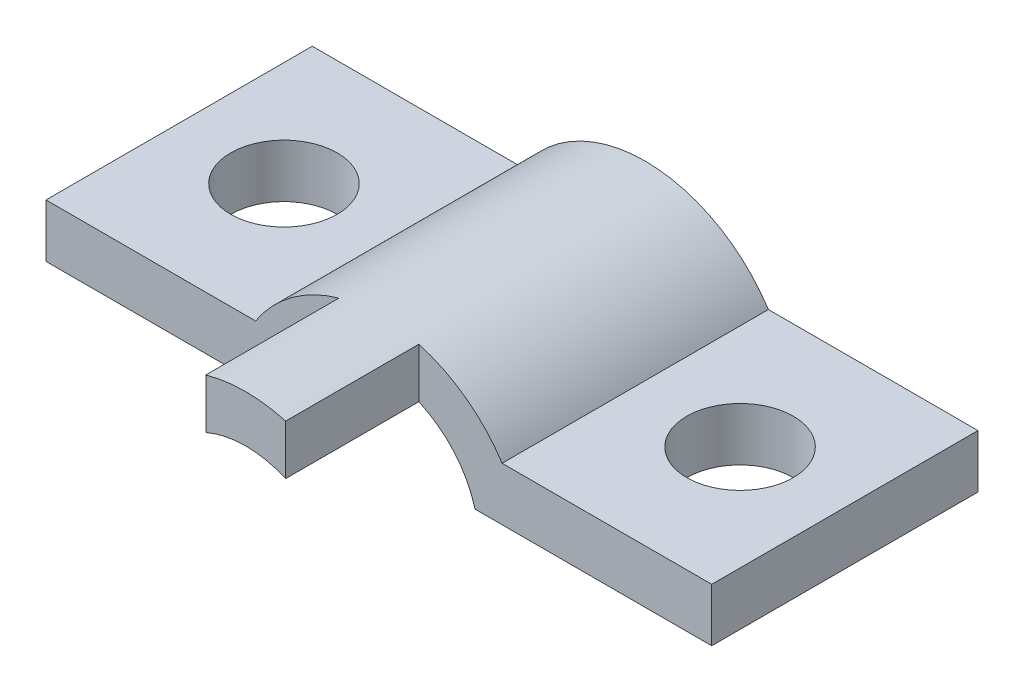
SolidWorks part; units mm, degrees
ref_plane "前视基准面" through (0, 0, 0) normal (0, 0, 1) x (1, 0, 0)
ref_plane "上视基准面" through (0, 0, 0) normal (0, 1, 0) x (1, 0, 0)
ref_plane "右视基准面" through (0, 0, 0) normal (1, 0, 0) x (0, 0, -1)
sketch "草图1" plane through (0, 0, 0) normal (0, 0, 1) x (1, 0, 0)
  line L0 (7.2284, 4) -> (25, 4)
  line L1 (-25, 8) -> (-9.2569, 8)
  line L3 (-25, 4) -> (-25, 8)
  line L4 (25, 8) -> (25, 4)
  line L8 (-25, 4) -> (-7.2284, 4)
  line L9 (25, 8) -> (9.2569, 8)
  arc A0 (7.2284, 4) -> (-7.2284, 4) centre (0, 2) ccw
  arc A1 (9.2569, 8) -> (-9.2569, 8) centre (0, 2) ccw
  dimension "D1" = 4
extrude "拉伸5" add sketch "草图1" along normal blind 30
sketch "草图5" plane through (0, 4, 0) normal (0, -1, 0) x (1, 0, 0)
  line L0 (-25, 30) -> (-25, 0) construction
  line L1 (-25, 20) -> (-3, 20)
  line L2 (-25, 20) -> (-25, 30)
  line L3 (-25, 30) -> (-3, 30)
  line L4 (3, 30) -> (25, 30)
  line L5 (-3, 20) -> (-3, 30)
  line L6 (7.2284, 30) -> (-7.2284, 30) construction
  line L8 (3, 30) -> (3, 20)
  line L9 (3, 20) -> (25, 20)
  line L10 (25, 30) -> (25, 20)
  dimension "D2" = 6
  dimension "D3" = 3
extrude "拉伸7" cut sketch "草图5" against normal through all
sketch "草图6" plane through (0, 8, 0) normal (0, 1, 0) x (1, 0, 0)
  circle A0 centre (-17.1284, -10) radius 4
  circle A1 centre (17.1284, -10) radius 4
extrude "拉伸8" cut sketch "草图6" against normal through all
